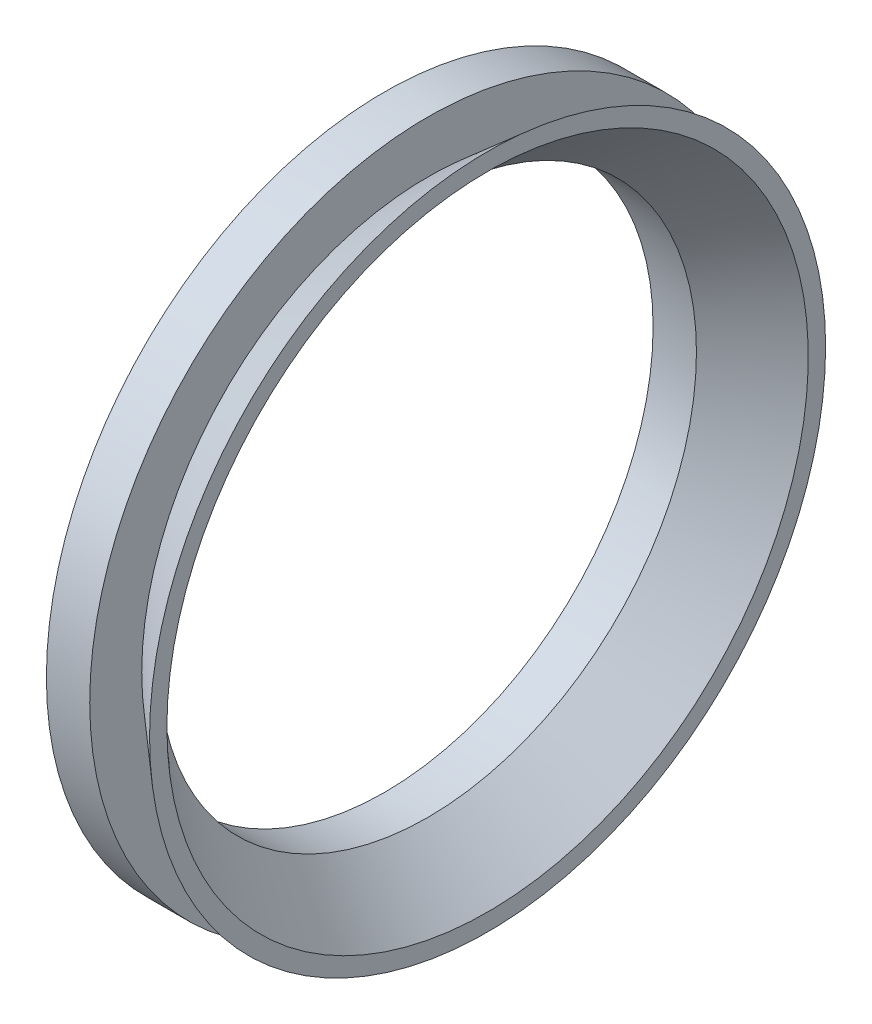
from build123d import *


with BuildPart() as part:
    # 草图1 → 旋转1 (revolve)
    with BuildSketch(Plane.XY, mode=Mode.PRIVATE) as revolve_1_sk:
        Polygon((0, 0), (2.5, 0), (5.951105222, 3), (5.951105222, 4), (2.5, 1), (2.5, 4), (0, 4), align=None)
    revolve(revolve_1_sk.sketch.rotate(Axis((-6.870284449, -15.5, 0), (1, 0, 0)), 90), axis=Axis((-6.870284449, -15.5, 0), (1, 0, 0)))


solid = part.part
